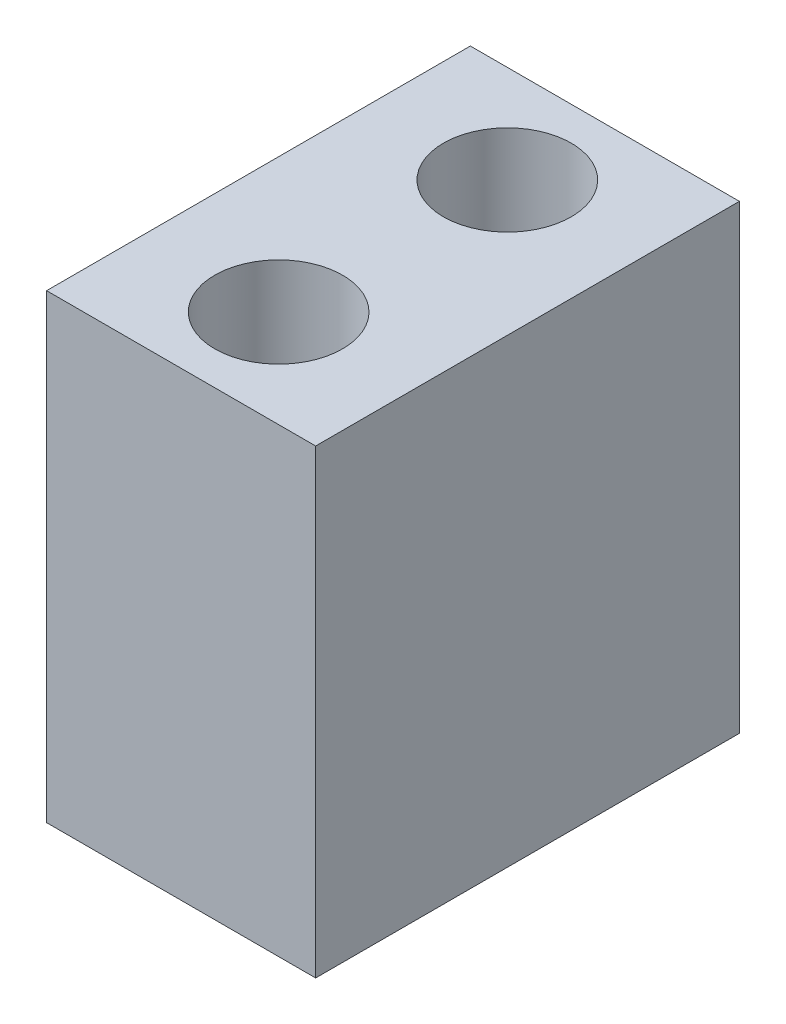
from build123d import *

# Parameters (mm, degrees)
SKETCH2_W           = 80
SKETCH2_H           = 126
SKETCH2_R           = 19
BOSS_EXTRUDE1_DEPTH = 68.5


with BuildPart() as part:
    # Sketch2 → Boss-Extrude1 (new, symmetric)
    with BuildSketch(Plane(origin=(0, 0, 0), x_dir=(1, 0, 0), z_dir=(0, 1, 0))):
        Rectangle(SKETCH2_W, SKETCH2_H)
        with Locations(Location((0, 34, 0), (0, 0, 270))):
            Circle(SKETCH2_R, mode=Mode.SUBTRACT)
        with Locations(Location((0, -34, 0), (0, 0, 270))):
            Circle(SKETCH2_R, mode=Mode.SUBTRACT)
    extrude(amount=BOSS_EXTRUDE1_DEPTH, both=True)


solid = part.part
